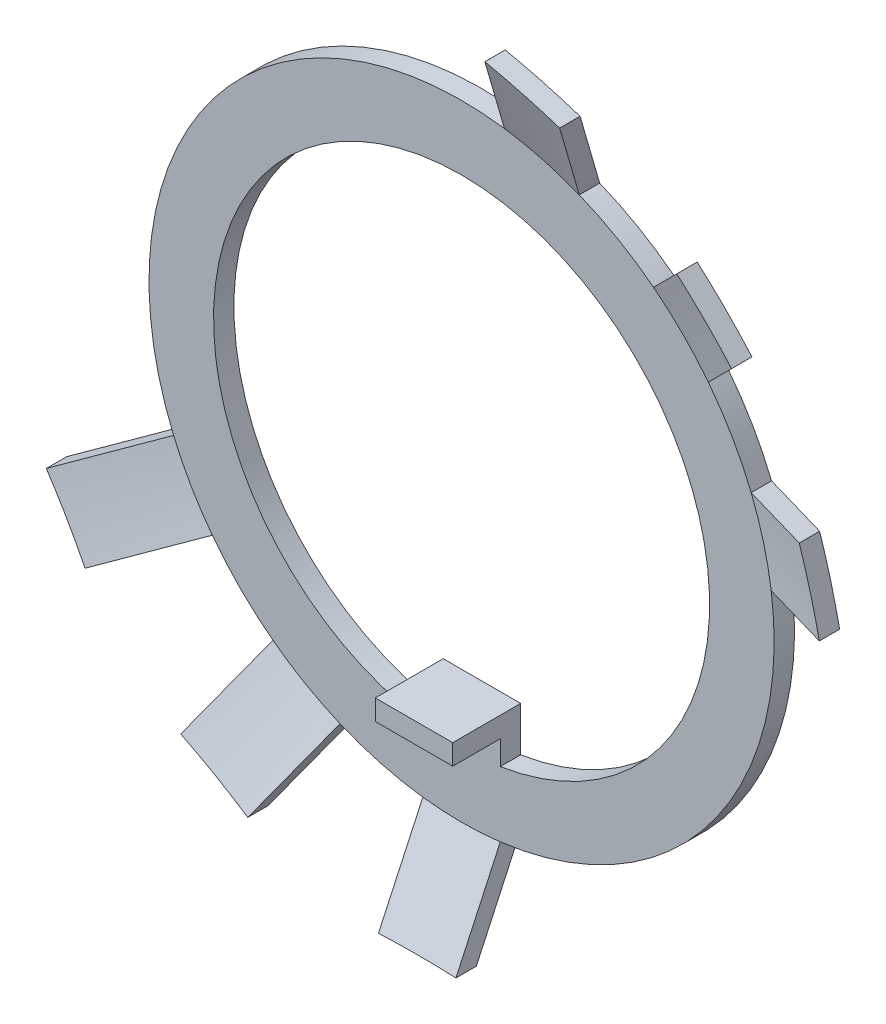
from build123d import *

# Parameters (mm, degrees)
CUT_EXTRUDE_START   = -2e-06
SKETCH_3_OUTSIDE_W  = 78.998
SKETCH_3_OUTSIDE_H  = 78.998
CUT_EXTRUDE_2_DEPTH = 4.764157
SKETCH_4_W          = 5.7
SKETCH_4_H          = 1.5
EXTRUDE_1_DEPTH     = 5


with BuildPart() as part:
    # 草图2 → Revolve 544 (revolve)
    with BuildSketch(Plane(origin=(0, 0, 0), x_dir=(0, 0, -1), z_dir=(1, 0, 0))):
        Polygon((-3.264153607, 30), (0, 23), (0, 0), (-1.5, 0), (-1.5, 23), (-4.764153607, 30), align=None)
    revolve(axis=Axis((0, 0, 0), (0, 0, 1)))

    # 草图3 outside → 切除-拉伸2 (cut)
    # profile 1 of 2: a face of its own
    with BuildSketch(Plane.XY.offset(CUT_EXTRUDE_START)):
        Rectangle(SKETCH_3_OUTSIDE_W, SKETCH_3_OUTSIDE_H)
        with BuildLine():
            Line((-2.85, -22.822740852), (-2.85, -29.864318174))
            Line((-2.85, -29.864318174), (2.85, -29.864318174))
            Line((2.85, -29.864318174), (2.85, -22.822740852))
            ThreePointArc((2.85, -22.822740852), (18.247126827, -14.001512867), (22.782709094, 3.154071389))
            Line((22.782709094, 3.154071389), (29.584350487, 4.976565708))
            Line((29.584350487, 4.976565708), (28.10908193, 10.482342917))
            Line((28.10908193, 10.482342917), (21.307440537, 8.659848599))
            ThreePointArc((21.307440537, 8.659848599), (19.918584287, 11.5), (18.153369148, 14.122860495))
            Line((18.153369148, 14.122860495), (23.132516223, 19.10200757))
            Line((23.132516223, 19.10200757), (19.10200757, 23.132516223))
            Line((19.10200757, 23.132516223), (14.122860495, 18.153369148))
            ThreePointArc((14.122860495, 18.153369148), (11.5, 19.918584287), (8.659848599, 21.307440537))
            Line((8.659848599, 21.307440537), (10.482342917, 28.10908193))
            Line((10.482342917, 28.10908193), (4.976565708, 29.584350487))
            Line((4.976565708, 29.584350487), (3.154071389, 22.782709094))
            ThreePointArc((3.154071389, 22.782709094), (-18.247126827, 14.001512867), (-21.190073362, -8.943198025))
            Line((-21.190073362, -8.943198025), (-27.288258205, -12.463986686))
            Line((-27.288258205, -12.463986686), (-24.438258205, -17.400331488))
            Line((-24.438258205, -17.400331488), (-18.340073362, -13.879542827))
            ThreePointArc((-18.340073362, -13.879542827), (-16.263455967, -16.263455967), (-13.879542827, -18.340073362))
            Line((-13.879542827, -18.340073362), (-17.400331488, -24.438258205))
            Line((-17.400331488, -24.438258205), (-12.463986686, -27.288258205))
            Line((-12.463986686, -27.288258205), (-8.943198025, -21.190073362))
            ThreePointArc((-8.943198025, -21.190073362), (-5.952838037, -22.216294005), (-2.85, -22.822740852))
        make_face(mode=Mode.SUBTRACT)
    # profile 2 of 2: a face of its own
    with BuildSketch(Plane.XY.offset(CUT_EXTRUDE_START)):
        with BuildLine():
            Line((2.85, -18.0260922), (2.85, -14.75))
            Line((2.85, -14.75), (-2.85, -14.75))
            Line((-2.85, -14.75), (-2.85, -18.0260922))
            ThreePointArc((-2.85, -18.0260922), (0, 18.25), (2.85, -18.0260922))
        make_face()
    extrude(amount=CUT_EXTRUDE_2_DEPTH, mode=Mode.SUBTRACT)

    # 草图4 → 凸台-拉伸1 (add)
    with BuildSketch(Plane.XY):
        with Locations((0, -15.5)):
            Rectangle(SKETCH_4_W, SKETCH_4_H)
    extrude(amount=EXTRUDE_1_DEPTH)


solid = part.part
